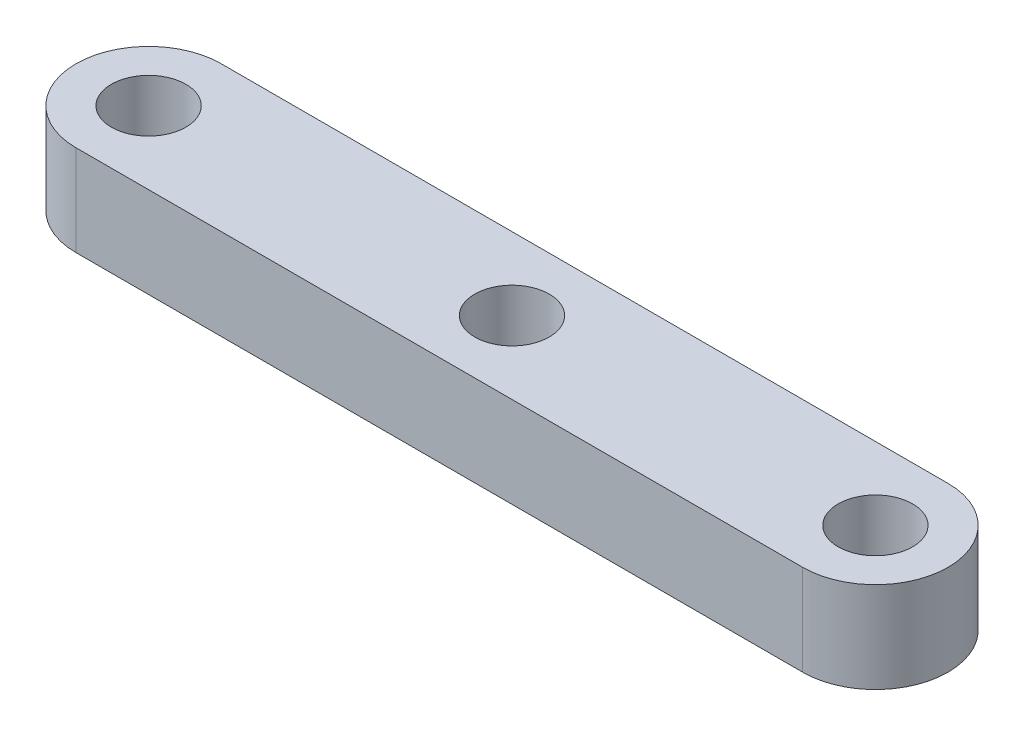
from build123d import *

# Parameters (mm, degrees)
SKETCH1_R           = 2.9
BOSS_EXTRUDE1_DEPTH = 6.35
BOSS_EXTRUDE2_START = -6.35
SKETCH2_R           = 2.9
SKETCH2_R_2         = 2.6035
BOSS_EXTRUDE2_DEPTH = 6.35
SKETCH2_2_R         = 2.6035
CUT_EXTRUDE1_DEPTH  = 57.468604552


with BuildPart() as part:
    # Sketch1 → Boss-Extrude1 (new body)
    with BuildSketch(Plane(origin=(0, 0, 0), x_dir=(1, 0, 0), z_dir=(0, 1, 0))):
        with BuildLine():
            Line((0, 5.08), (50.8, 5.08))
            ThreePointArc((50.8, 5.08), (55.88, 0), (50.8, -5.08))
            Line((50.8, -5.08), (0, -5.08))
            ThreePointArc((0, -5.08), (-5.08, 0), (0, 5.08))
        make_face()
        with Locations(Location((0, 0, 0), (0, 0, 270))):
            Circle(SKETCH1_R, mode=Mode.SUBTRACT)
        with Locations(Location((50.8, 0, 0), (0, 0, 270))):
            Circle(SKETCH1_R, mode=Mode.SUBTRACT)
    extrude(amount=BOSS_EXTRUDE1_DEPTH)

    # Sketch2 → Boss-Extrude2 (add)
    # profile 1 of 3: a face of its own
    with BuildSketch(Plane(origin=(0, 6.35, 0), x_dir=(1, 0, 0), z_dir=(0, 1, 0)).offset(BOSS_EXTRUDE2_START)):
        Circle(SKETCH2_R)
        with Locations(Location((0, 0, 0), (0, 0, 270))):
            Circle(SKETCH2_R_2, mode=Mode.SUBTRACT)
    # profile 2 of 3: a face of its own
    with BuildSketch(Plane(origin=(0, 6.35, 0), x_dir=(1, 0, 0), z_dir=(0, 1, 0)).offset(BOSS_EXTRUDE2_START)):
        with Locations((50.8, 0)):
            Circle(SKETCH2_R)
        with Locations(Location((50.8, 0, 0), (0, 0, 270))):
            Circle(SKETCH2_R_2, mode=Mode.SUBTRACT)
    # profile 3 of 3: a face of its own
    with BuildSketch(Plane(origin=(0, 6.35, 0), x_dir=(1, 0, 0), z_dir=(0, 1, 0)).offset(BOSS_EXTRUDE2_START)):
        with Locations((25.4, 0)):
            Circle(SKETCH2_R_2)
    extrude(amount=BOSS_EXTRUDE2_DEPTH)

    # Sketch2<2> → Cut-Extrude1 (cut, through all)
    with BuildSketch(Plane(origin=(0, 6.35, 0), x_dir=(1, 0, 0), z_dir=(0, 1, 0))):
        with Locations(Location((25.4, 0, 0), (0, 0, 270))):
            Circle(SKETCH2_2_R)
    extrude(amount=-CUT_EXTRUDE1_DEPTH, mode=Mode.SUBTRACT)


solid = part.part
